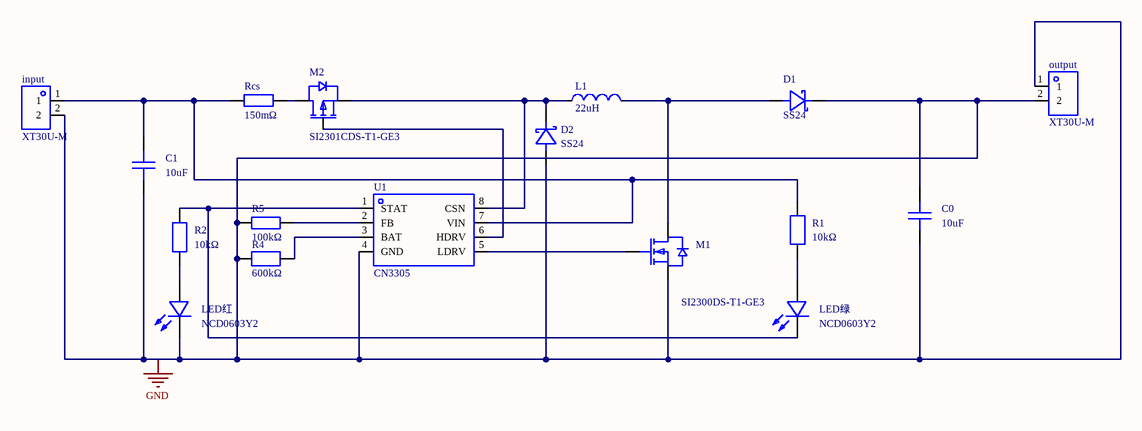
[diagram p0: MISC51207-3.schdoc]
# Altium project MISC51207-2.PrjPcb
1 sheet, 17 parts. Net scope: global (net labels, ports and power ports of the same name join across sheets).
Board file: MISC51207.pcbdoc

## Sheet MISC51207-3.schdoc
size 297 x 209 mm; Version: V1.0; @Project Name: MISC51207; @Update Date: 2026-03-15; @Create Date: 2026-03-15; @Board Name: MISC51207; @Create Time: 19:09:47; @Page Count: 1; @Page No: 1; @Schematic Name: MISC51207; @Update Time: 19:09:47; Size: A4

### Parts
C0  10uF  [C0805]
C1  10uF  [C0805]
D1  SS24  [SMA_L4.3-W2.6-LS5.0-FD]
D2  SS24  [SMA_L4.3-W2.6-LS5.0-FD]
input  XT30U-M  [CONN-TH_XT30U-M]
L1  22uH  [IND-SMD_L7.0-W6.6_FXL0630]
LED红  NCD0603Y2  [LED0603-RD]
LED绿  NCD0603Y2  [LED0603-RD]
M1  SI2300DS-T1-GE3  [SOT-23-3_L2.9-W1.6-P1.90-LS2.8-BR]
M2  SI2301CDS-T1-GE3  [SOT-23-3_L3.0-W1.7-P0.95-LS2.9-BR]
output  XT30U-M  [CONN-TH_XT30U-M]
R1  10kΩ  [R0805]
R2  10kΩ  [R0805]
R4  600kΩ  [RES-TH_BD3.7-L8.7-P12.8-D0.8]
R5  100kΩ  [RES-TH_BD2.7-L6.2-P10.20-D0.4]
Rcs  150mΩ  [R1206]
U1  CN3305  [SOP-8_L4.9-W3.9-P1.27-LS6.0-BL-1]

### Nets
GND: C0.1 C0.2 C1.1 D1.2(K) D2.1(A) input.2 LED红.1(K) M1.2(S) output.1 output.2 R4.1 R5.1 U1.4(GND)
NetC1_2: C1.2 input.1 R1.2 Rcs.1 U1.7(VIN)
NetD1_1: D1.1(A) L1.2 M1.3(D)
NetD2_2: D2.2(K) L1.1 M2.2(S) U1.8(CSN)
NetLED红_2: LED红.2(A) R2.1
NetLED绿_1: LED绿.1(K) R2.2 U1.1(STAT)
NetLED绿_2: LED绿.2(A) R1.1
NetM1_1: M1.1(G) U1.5(LDRV)
NetM2_1: M2.1(G) U1.6(HDRV)
NetM2_3: M2.3(D) Rcs.2
NetR4_2: R4.2 U1.3(BAT)
NetR5_2: R5.2 U1.2(FB)

### Notes on the sheet
- 2026-03-15
- 原理图
- P1
- 版本
- 尺寸
- A4
- 页    1    共    1

### Library data of the parts
C0 C1 = CGA0805X5R106K250MT: 容值:10uF;精度:±10%;额定电压:25V;温度系数:X5R;; Manufacturer: HRE(芯声); AddInBom: yes; ModelId: 1ba041120af144c991958decab20d2410819f05c4eef4c71ace90d822a990e87; ModelName: C0805_L2.0-W1.3-H1.3; ModelTransform: 78.74,51.181,0,0,0,0,0,0.0005,0; Tolerance: ±10%; Voltage Rating: 25V; Temperature Coefficient: X5R; Symbol: CGA0805X5R106K250MT; Device: CGA0805X5R106K250MT; LCSC Part Name: 10uF ±10% 25V; SupplierPart: C6119887; ManufacturerPart: CGA0805X5R106K250MT; Supplier Footprint: 0805; JLCPCB Part Class: Extended Part; Datasheet: https://item.szlcsc.com/datasheet/CGA0805X5R106K250MT/7062593.html; Supplier: LCSC; ConvertToPcb: yes; FootprintName: C0805; Value: 10uF
D1 D2 = SS24_C7420362: 二极管配置:独立式;正向压降(Vf):550mV@2A;直流反向耐压(Vr):40V;整流电流:2A;; Manufacturer: R+O(宏嘉诚); AddInBom: yes; ModelId: 7e24bebe6cd74171ae8c9de6fc5b78aa0819f05c4eef4c71ace90d822a990e87; ModelTransform: 198.4248,103.5431,0,180,0,0,-0.001,0,0; Diode Configuration: 独立式; Voltage - DC Reverse(Vr): 40V; Current - Rectified: 2A; Reverse Leakage Current (Ir): 200uA@40V; Operating Junction Temperature Range: -55℃~+150℃; Non-Repetitive Peak Forward Surge Current: 50A; Symbol: SS24_C7420362; Device: SS24_C7420362; LCSC Part Name: 电压:40V 电流:2A; SupplierPart: C7420362; ManufacturerPart: SS24; Supplier Footprint: SMA(DO-214AC); JLCPCB Part Class: Extended Part; Datasheet: https://item.szlcsc.com/datasheet/SS24/8397184.html; Supplier: LCSC; ConvertToPcb: yes; FootprintName: SMA_L4.3-W2.6-LS5.0-FD; ModelName: SMA_L4.3-W2.6-LS5.0-FD; Voltage - Forward(Vf@If): 550mV@2A
input output = XT30U-M: 模型插头轻量版锂电池插头; Manufacturer: AMASS(艾迈斯); AddInBom: yes; ModelId: c4d22a730da840da8ffa3a8fc42a4c700819f05c4eef4c71ace90d822a990e87; ModelTransform: 401.574,204.724,0,180,0,0,-0.005,0,-118.11; Connector type: 插头; interface form: 公头; Symbol: XT30U-M; Device: XT30U-M; LCSC Part Name: AMASS(艾迈斯)航模插头电调机插座锂电池连接器 轻量版 公头XT30U-M; SupplierPart: C99101; ManufacturerPart: XT30U-M; Supplier Footprint: -; JLCPCB Part Class: Extended Part; Datasheet: https://item.szlcsc.com/datasheet/XT30U-M/100314.html; Supplier: LCSC; ConvertToPcb: yes; FootprintName: CONN-TH_XT30U-M; ModelName: CONN-TH_XT30U-M; colour: 黄色
L1 = FXL0630-220-M: 电感值:22uH;精度:±20%;额定电流:2.5A;饱和电流(Isat):3A;类型:一体成型电感;; Manufacturer: cjiang(长江微电); AddInBom: yes; ModelId: 6712504104d74f0ca01cd7d0df9965b70819f05c4eef4c71ace90d822a990e87; ModelName: IND-SMD_L7.0-W6.6-H2.8_FXL0630; ModelTransform: 275.59,259.842,0,0,0,0,0,0,0; Tolerance: ±20%; Current Rating: 2.5A; Current - Saturation(Isat): 3A; DC Resistance(DCR): 200mΩ; Type: 一体成型电感; Symbol: FXL0630-220-M; Device: FXL0630-220-M; LCSC Part Name: 22uH ±20% 3A; SupplierPart: C177244; ManufacturerPart: FXL0630-220-M; Supplier Footprint: SMD,7x6.6mm; JLCPCB Part Class: Extended Part; Datasheet: https://item.szlcsc.com/datasheet/FXL0630-220-M/188636.html; Supplier: LCSC; ConvertToPcb: yes; FootprintName: IND-SMD_L7.0-W6.6_FXL0630; Value: 22uH
LED红 LED绿 = NCD0603Y2: 发光颜色:黄色;正向电压(VF):1.6V~2.6V;功率:65mW;正向电流:20mA;主波长:586nm~595nm;透镜颜色:无色透明透镜;发光强度:100mcd~220mcd;发光角度:130°;工作温度:-30℃~+85℃;; Manufacturer: 国星光电; Symbol: FC-1608YXK-585F08; AddInBom: yes; ModelId: 1f0d29a91be547639d425604e9b96ebb0819f05c4eef4c71ace90d822a990e87; ModelTransform: 63.7794,32.283,0,0,0,0,0,0,0; Emitted Color: 黄色; Power Dissipation: 65mW; Forward Current: 20mA; Lens Color: 无色透明透镜; Viewing Angle: 130°; Device: NCD0603Y2; LCSC Part Name: NCD0603Y2; SupplierPart: C89811; ManufacturerPart: NCD0603Y2; Supplier Footprint: 0603; JLCPCB Part Class: Extended Part; Datasheet: https://atta.szlcsc.com/upload/public/pdf/source/20200820/C89811_7FE84B429B6BCA3E113B125EE1452576.pdf; Supplier: LCSC; ConvertToPcb: yes; FootprintName: LED0603-RD; ModelName: LED0603-RD; Forward Voltage (VF): 1.6V~2.6V; Dominant Wavelength: 586nm~595nm; Luminous Intensity: 100mcd~220mcd; Operating Temperature: -30℃~+85℃
M1 = SI2300DS-T1-GE3: 数量:1个N沟道;漏源电压(Vdss):30V;连续漏极电流(Id):3.6A;导通电阻(RDS(on)):68mΩ@4.5V,2.9A;耗散功率(Pd):1.1W;阈值电压(Vgs(th)):1.5V;; Manufacturer: VISHAY(威世); AddInBom: yes; ModelId: 89cb27a44ab2466697082bb9fd73a7d00819f05c4eef4c71ace90d822a990e87; ModelName: SOT-23-3L_L2.9-W1.6-H1.1-LS2.8-P0.95; ModelTransform: 114.173,110.236,0,90,0,0,0,0,0; Number: 1个N沟道; Drain to Source Voltage: 30V; Current - Continuous Drain(Id): 3.6A; Pd - Power Dissipation: 1.1W; Gate Threshold Voltage (Vgs(th)): 1.5V; Gate Charge(Qg): 6.5nC@10V; Input Capacitance(Ciss): 320pF@15V; Reverse Transfer Capacitance (Crss@Vds): 19pF@15V; Symbol: SI2300DS-T1-GE3; Device: SI2300DS-T1-GE3; LCSC Part Name: 1个N沟道 耐压:30V 电流:3.6A; SupplierPart: C72271; ManufacturerPart: SI2300DS-T1-GE3; Supplier Footprint: SOT-23; JLCPCB Part Class: Extended Part; Datasheet: https://item.szlcsc.com/datasheet/SI2300DS-T1-GE3/73380.html; Supplier: LCSC; ConvertToPcb: yes; FootprintName: SOT-23-3_L2.9-W1.6-P1.90-LS2.8-BR; RDS(on): 68mΩ@4.5V,2.9A; Operating Temperature: -55℃~+150℃
M2 = SI2301CDS-T1-GE3: 数量:1个P沟道;漏源电压(Vdss):20V;连续漏极电流(Id):3.1A;导通电阻(RDS(on)):142mΩ@2.5V,2.7A;耗散功率(Pd):1.6W;阈值电压(Vgs(th)):1V@250uA;; Manufacturer: VISHAY(威世); AddInBom: yes; ModelId: 89cb27a44ab2466697082bb9fd73a7d00819f05c4eef4c71ace90d822a990e87; ModelName: SOT-23-3L_L2.9-W1.6-H1.1-LS2.8-P0.95; ModelTransform: 114.173,110.236,0,90,0,0,0,0,0; Number: 1个P沟道; Drain to Source Voltage: 20V; Current - Continuous Drain(Id): 3.1A; Pd - Power Dissipation: 1.6W; Gate Charge(Qg): 10nC@4.5V; Input Capacitance(Ciss): 405pF; Reverse Transfer Capacitance (Crss@Vds): 55pF; Output Capacitance(Coss): 75pF; Symbol: SI2301CDS-T1-GE3; Device: SI2301CDS-T1-GE3; LCSC Part Name: 1个P沟道 耐压:20V 电流:3.1A; SupplierPart: C10487; ManufacturerPart: SI2301CDS-T1-GE3; Supplier Footprint: SOT-23; JLCPCB Part Class: Basic Part; Datasheet: https://item.szlcsc.com/datasheet/SI2301CDS-T1-GE3/11030.html; Supplier: LCSC; ConvertToPcb: yes; FootprintName: SOT-23-3_L3.0-W1.7-P0.95-LS2.9-BR; RDS(on): 142mΩ@2.5V,2.7A; Gate Threshold Voltage (Vgs(th)): 1V@250uA; Operating Temperature: -55℃~+150℃; Type: P沟道
R1 R2 = FRR0805J103 TS: 电阻类型:厚膜电阻;阻值:10kΩ;精度:±5%;功率:125mW;工作电压:150V;温度系数:±100ppm/℃;; Manufacturer: FOJAN(富捷); AddInBom: yes; ModelId: 37a81e68749a4138bd2dfa6897b24b850819f05c4eef4c71ace90d822a990e87; ModelName: R0805_L2.0-W1.3-H0.6; ModelTransform: 78.74,51.181,0,0,0,0,0,-0.0005,0; Tolerance: ±5%; Power(Watts): 125mW; Voltage-Supply(Max): 150V; Symbol: FRR0805J103 TS; Device: FRR0805J103 TS; LCSC Part Name: 厚膜电阻 0805 10KΩ ±5% 125mW; SupplierPart: C49196826; ManufacturerPart: FRR0805J103 TS; Supplier Footprint: 0805; JLCPCB Part Class: Extended Part; Datasheet: https://item.szlcsc.com/datasheet/FRR0805J103%2520TS/51599074.html; Supplier: LCSC; ConvertToPcb: yes; FootprintName: R0805; Type: 厚膜电阻; Value: 10kΩ; Temperature Coefficient: ±100ppm/℃; Operating Temperature: -55℃~+155℃
R4 = RN60D6003FB14: 电阻类型:金属膜电阻;阻值:600kΩ;精度:±1%;功率:250mW;温度系数:±100ppm/℃;; Manufacturer: VISHAY(威世); AddInBom: yes; ModelId: 2d8dc72bb74d4892b4dab800bb220e010819f05c4eef4c71ace90d822a990e87; ModelTransform: 535.432,146.06262,0,0,0,0,-0.003,-0.004,-196.85; Tolerance: ±1%; Power(Watts): 250mW; Symbol: RN60D6003FB14; Device: RN60D6003FB14; LCSC Part Name: 金属膜电阻 600kΩ ±1% 250mW; SupplierPart: C1395381; ManufacturerPart: RN60D6003FB14; Supplier Footprint: 插件,D3.7xL8.7mm; JLCPCB Part Class: Extended Part; Datasheet: https://item.szlcsc.com/datasheet/RN60D6003FB14/1485673.html; Supplier: LCSC; ConvertToPcb: yes; FootprintName: RES-TH_BD3.7-L8.7-P12.8-D0.8; ModelName: RES-TH_BD3.7-L8.7-P12.8-D0.8; Type: 金属膜电阻; Value: 600kΩ; Temperature Coefficient: ±100ppm/℃; Operating Temperature: -65℃~+175℃
R5 = MF1/4W-100K±1%-OT26: 电阻类型:金属膜电阻;阻值:100kΩ;精度:±1%;功率:250mW;温度系数:±350ppm/℃;; Manufacturer: VO(翔胜); AddInBom: yes; ModelId: f91fbe0e2e6f409498f09f811e4616fe0819f05c4eef4c71ace90d822a990e87; ModelTransform: 417.322,106.221,0,0,0,0,0,0,-196.85; Tolerance: ±1%; Overload Voltage (Max): 250V; Power(Watts): 250mW; Symbol: MF1/4W-100K±1%-OT26; Device: MF1/4W-100K±1%-OT26; LCSC Part Name: 金属膜电阻 100kΩ ±1% 250mW; SupplierPart: C2843019; ManufacturerPart: MF1/4W-100K±1%-OT26; Supplier Footprint: 插件,D2.7xL6.2mm; JLCPCB Part Class: Extended Part; Datasheet: https://atta.szlcsc.com/upload/public/pdf/source/20200609/C601728_5AA4C0C8E12E11069DA2C3356F29D1F2.pdf; Supplier: LCSC; ConvertToPcb: yes; FootprintName: RES-TH_BD2.7-L6.2-P10.20-D0.4; ModelName: RES-TH_BD2.7-L6.2-P10.20-D0.4; Type: 金属膜电阻; Value: 100kΩ; Temperature Coefficient: ±350ppm/℃; Operating Temperature Range: -55℃~+155℃
Rcs = 1206W4F150LT5E: 电阻类型:厚膜电阻;阻值:150mΩ;精度:±1%;功率:250mW;工作电压:200V;温度系数:±800ppm/℃;; Manufacturer: UNI-ROYAL(厚声); AddInBom: yes; ModelId: 89a1f13db2384da588040e0b3c55bf660819f05c4eef4c71ace90d822a990e87; ModelName: R1206_L3.2-W1.6-H0.6; ModelTransform: 125.984,62.992,0,0,0,0,0,0,0; Tolerance: ±1%; Power(Watts): 250mW; Voltage-Supply(Max): 200V; Symbol: 1206W4F150LT5E; Device: 1206W4F150LT5E; LCSC Part Name: 150mΩ ±1% 250mW 厚膜电阻; SupplierPart: C37936; ManufacturerPart: 1206W4F150LT5E; Supplier Footprint: 1206; JLCPCB Part Class: Extended Part; Datasheet: https://item.szlcsc.com/datasheet/1206W4F150LT5E/38917.html; Supplier: LCSC; ConvertToPcb: yes; FootprintName: R1206; Type: 厚膜电阻; Value: 150mΩ; Temperature Coefficient: ±800ppm/℃; Operating Temperature: -55℃~+155℃
U1 = CN3305: 工作电压:2.7V~6.5V;最大充电电流:-;电池类型:磷酸铁锂电池；铅酸电池；锂电池;; Manufacturer: CONSONANCE(上海如韵); Symbol: CN3305_C3034875; AddInBom: yes; ModelId: 75c24a7891ee4dd6bdac16a7163ff87e0819f05c4eef4c71ace90d822a990e87; ModelTransform: 192.913,236.22,0,0,0,0,0,0,0; The Chip Type: 充电芯片; Charging Saturation Voltage: 1.205V; Battery Temperature Detection: 不支持; Supply Current (Iq): 360uA; Device: CN3305; LCSC Part Name: 停产 PFM升压型多节电池充电控制集成电路 停产; SupplierPart: C3034875; ManufacturerPart: CN3305; Supplier Footprint: SOP-8; JLCPCB Part Class: Extended Part; Datasheet: https://item.szlcsc.com/datasheet/CN3305/3581080.html; Supplier: LCSC; ConvertToPcb: yes; FootprintName: SOP-8_L4.9-W3.9-P1.27-LS6.0-BL-1; ModelName: SOP-8_L4.9-W3.9-P1.27-LS6.0-BL-1; Voltage - Supply: 2.7V~6.5V; Charge Current - Max: -; Type of Battery: 磷酸铁锂电池；铅酸电池；锂电池; Operating Temperature: -40℃~+85℃; 0V Battery Charge: 不支持